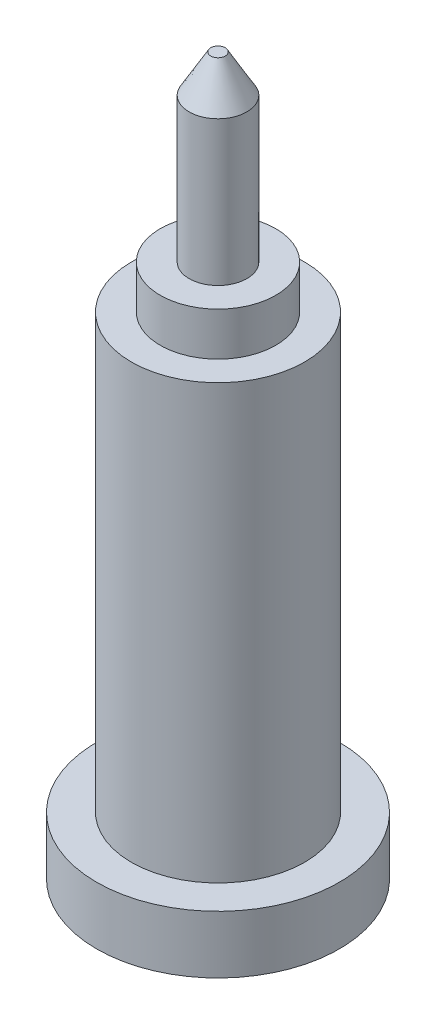
SolidWorks part; units mm, degrees
ref_plane "Front Plane" through (0, 0, 0) normal (0, 0, 1) x (1, 0, 0)
ref_plane "Top Plane" through (0, 0, 0) normal (0, 1, 0) x (1, 0, 0)
ref_plane "Right Plane" through (0, 0, 0) normal (1, 0, 0) x (0, 0, -1)
other "Configuration Table"
sketch "Sketch1" plane through (0, 0, 0) normal (0, 0, 1) x (1, 0, 0)
  line L0 (0, 0) -> (0, 87.6091) construction
  line L1 (-1.25, 0) -> (-4.2, 0)
  line L2 (-4.2, 0) -> (-4.2, 2)
  line L3 (-4.2, 2) -> (-3, 2)
  line L4 (-3, 2) -> (-3, 17)
  line L5 (-3, 17) -> (-2, 17)
  line L6 (-2, 17) -> (-2, 18.5)
  line L7 (-2, 18.5) -> (-1, 18.5)
  line L8 (-1, 18.5) -> (-1, 23.5)
  line L9 (-1, 23.5) -> (-0.25, 24.799)
  line L10 (-0.25, 24.799) -> (0, 24.799)
  line L11 (-1.25, 0) -> (-1.25, 6)
  line L12 (-1.25, 6) -> (0, 6)
  line L13 (0, 24.799) -> (0, 6)
  dimension "D1" = 2
  dimension "D2" = 3
  dimension "D3" = 4.2
  dimension "D4" = 15
  dimension "D5" = 2
  dimension "D6" = 1
  dimension "D7" = 0.25
  dimension "D8" = 30
  dimension "D9" = 1.5
  dimension "D10" = 5
  dimension "D11" = 6
  dimension "D12" = 2.5
revolve "Revolve1" add sketch "Sketch1" angle 360 about L0
